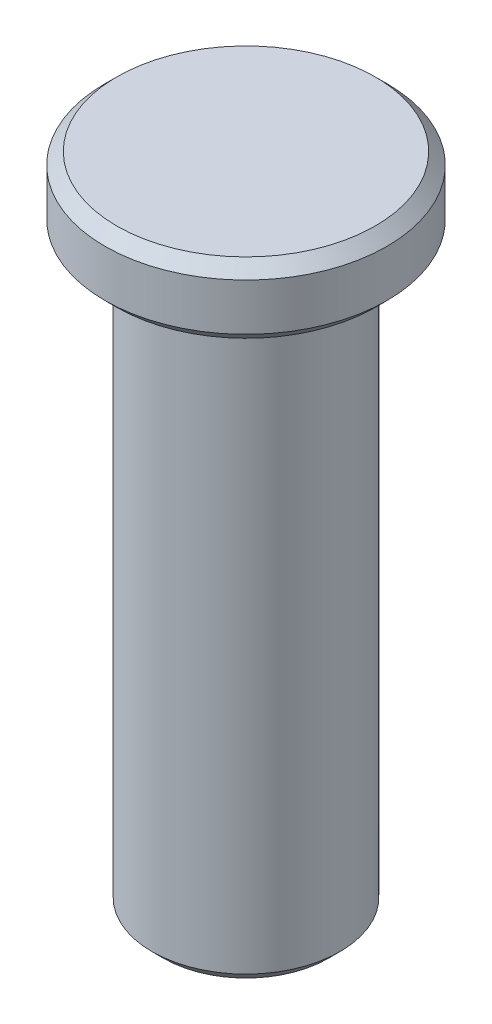
from build123d import *

# Parameters (mm, degrees)
SKETCH2_R           = 4
BOSS_EXTRUDE1_DEPTH = 25
SKETCH3_R           = 6
BOSS_EXTRUDE2_DEPTH = 3
CHAMFER1_SIZE       = 0.5


with BuildPart() as part:
    # Sketch2 → Boss-Extrude1 (new body)
    with BuildSketch(Plane(origin=(0, 0, 0), x_dir=(1, 0, 0), z_dir=(0, 1, 0))):
        with Locations(Location((0, 0, 0), (0, 0, 270))):
            Circle(SKETCH2_R)
    extrude(amount=BOSS_EXTRUDE1_DEPTH)

    # Sketch3 → Boss-Extrude2 (add)
    with BuildSketch(Plane(origin=(0, 25, 0), x_dir=(1, 0, 0), z_dir=(0, 1, 0))):
        with Locations(Location((0, 0, 0), (0, 0, 270))):
            Circle(SKETCH3_R)
    extrude(amount=BOSS_EXTRUDE2_DEPTH)

    # Chamfer1
    chamfer1_edges = [part.edges().sort_by_distance(p)[0] for p in [
        (0, 0, -4),
        (0, 25, -6),
        (0, 28, -6),
    ]]
    chamfer(chamfer1_edges, length=CHAMFER1_SIZE)


solid = part.part
